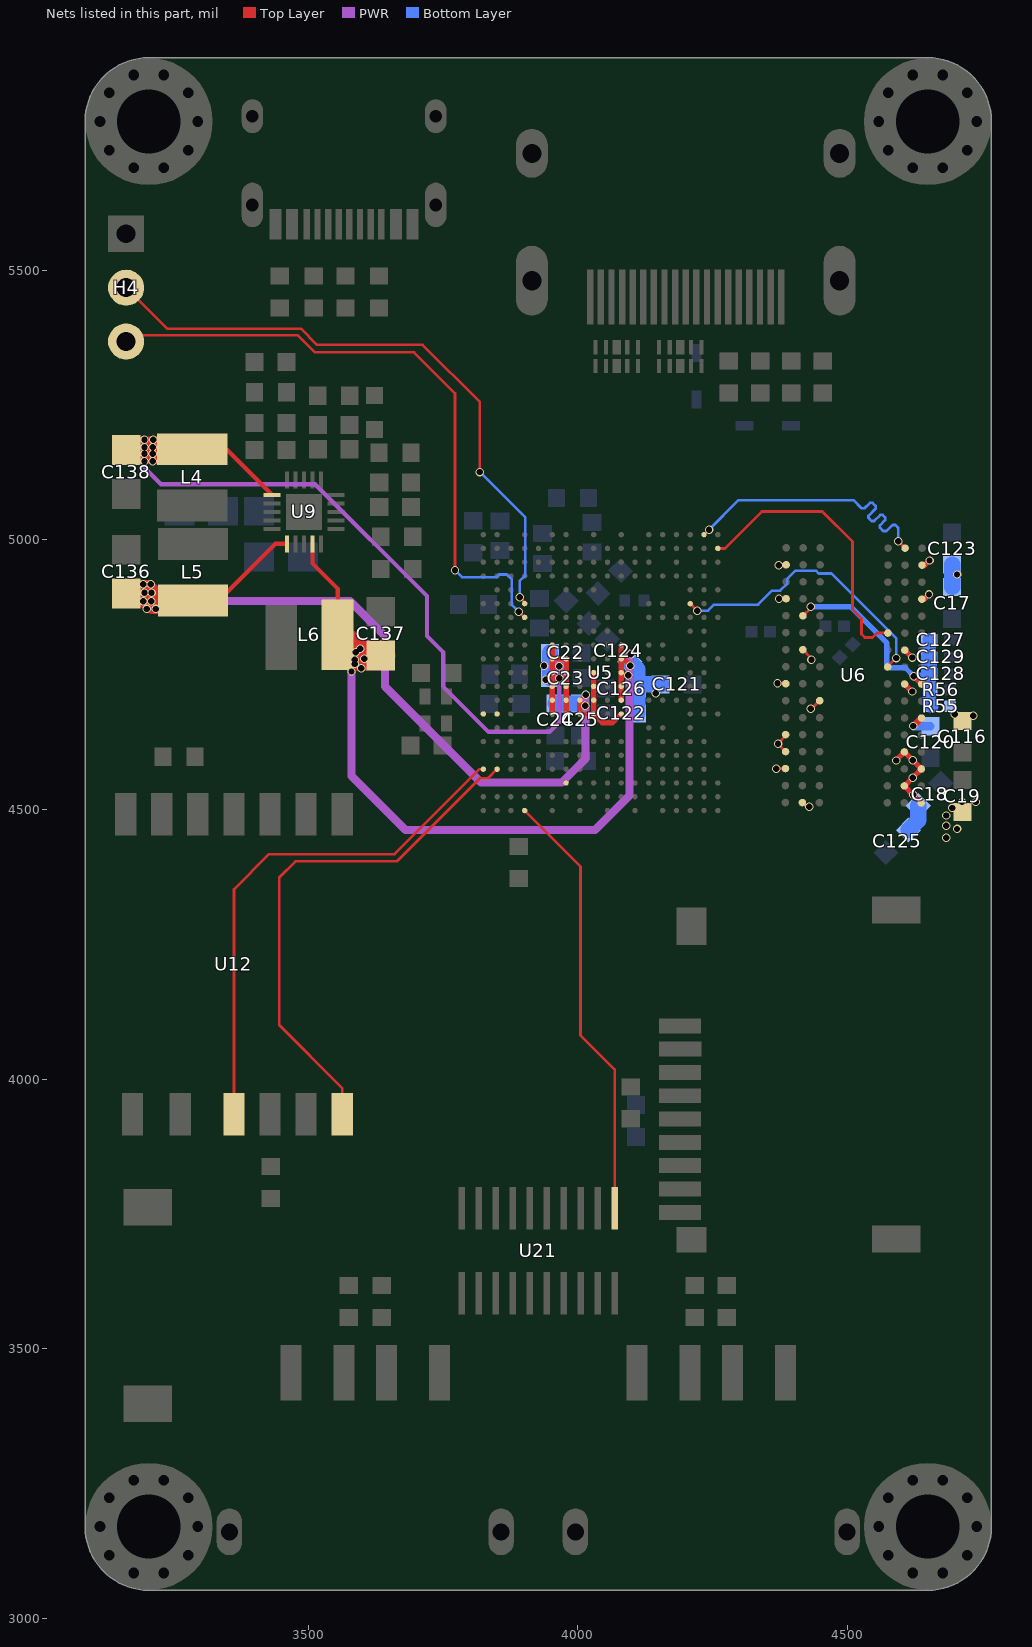
[diagram p0: the nets of this part, all layers, seen from the top]
# Altium PCB MISC105417.pcbdoc (part 5 of 5)
Units mil, origin at the board's own origin, x right, y up, seen from the top; angles counter-clockwise.
Board outline 1681.1 x 2842.52 mil, 4 copper layers (Top Layer, GND, PWR, Bottom Layer), stack 62.447 mil thick; 102 components, 152 nets, 737 pads, 611 vias.

## Via types
v1: diameter 15.7, hole 11.8, Top Layer to Bottom Layer, 611 vias

## Nets (pads, with @x,y where several pads share a name; then routed paths per layer and width w, separated by ;. In a path a pad name is that pad's centre, name@x,y a point inside that pad or via, vN(x,y) a via of type N, cw(c..) or ccw(c..) an arc to the next point about the centre after c; other vN are vias at no path point) (continued)
SRAS: U5.T16 U6.J3 | length 535
  Top Layer w5: U5.T16@4208.34,4881.95 4221.2,4869.09 v1(4221.2,4868.94) ; U6.J3@4574.64,4764.39 4574.64,4765.38 v1(4590.2,4780.94)
  Bottom Layer w5: v1(4221.2,4868.94) 4241.2,4868.94 4252.2,4879.94 4334.2,4879.94 4360.2,4905.94 4374.94,4905.94 4388.43,4919.43 4388.43,4928.16 4403.36,4943.09 4441.46,4943.09 4446.61,4937.94 4470.2,4937.94 4590.2,4817.94 v1(4590.2,4780.94)
SRST: U5.U21 U6.T2 | length 535
  Top Layer w5: U5.U21@4233.93,5009.91 4242.96,5018.94 v1(4243.2,5018.94) ; v1(4594.2,4997.94) 4606.84,4985.31 U6.T2@4606.84,4984.79
  Bottom Layer w5: v1(4243.2,5018.94) 4298.2,5073.94 4511.13,5073.94 4526.29,5058.78 4531.81,5058.78 4541.8,5068.78 4546.37,5068.78 4552.2,5062.94 4552.2,5057.94 4538.64,5044.37 4538.64,5041.19 4544.55,5035.28 4549.55,5035.28 4560.95,5046.69 4564.95,5046.69 4569.88,5041.76 4569.88,5036.82 4559.99,5026.93 4559.99,5022.87 4566.1,5016.75 4572.22,5016.75 4583.4,5027.93 4588.72,5027.93 4594.2,5022.45 v1(4594.2,4997.94)
STATE_LED: U5.G3
SVREF: C127.2 C128.2 C129.2 R55.2 R56.1 U6.H1 U6.M8 | length 464.4
  Top Layer w5: U6.M8@4417.44,4859.39 4432.2,4874.16 v1(4432.2,4875.94)
  Top Layer w10: v1@4623.29,4746.94 U6.H1@4637.54,4732.69
  Bottom Layer w10: v1(4432.2,4875.94) 4506.2,4875.94 4573.2,4808.94 4573.2,4770.94 4581.19,4762.96 4607.19,4762.96 v1(4623.2,4746.94)
  Bottom Layer w15: v1(4623.2,4746.94) 4646.51,4746.94 C128.2@4651.51,4751.94
  Bottom Layer w25: C128.2@4651.51,4751.94 4651.51,4696.36 R55.2@4655.93,4691.94 ; C129.2@4651.51,4782.94 C127.2@4651.51,4814.66
  Bottom Layer w30: C128.2@4651.51,4751.94 C129.2@4651.51,4782.94
SWE: U5.V20 U6.L3 | length 535
  Top Layer w5: U5.V20@4259.52,4984.31 4272.57,4984.31 4341.2,5052.94 4453.2,5052.94 4509.2,4996.94 4509.2,4870.94 4525.85,4854.29 4525.85,4825.29 4532.2,4818.94 4546.2,4818.94 4554.65,4827.39 U6.L3@4574.84,4827.39
TS_IRQ: U5.D1 U21.11 | length 806.7
  Top Layer w5: U5.D1@3901.25,4498.09 4004.86,4394.48 4004.86,4081.14 4068.17,4017.83 U21.11@4068.17,3760.55
UART0_RX: H4.3 U5.D15 | length 1184.8
  Top Layer w5: H4.3@3162,5368 3174,5380 3480,5380 3512,5348 3696,5348 3772,5272 v1(3772,4944) ; v1(3890.2,4866.94) 3890.67,4866.94 U5.D15@3901.25,4856.36
  Bottom Layer w5: v1(3772,4944) 3785,4931 3849,4931 3854,4936 3868,4936 3877.52,4926.48 3877.52,4879.63 v1(3890.2,4866.94)
UART0_TX: H4.2 U5.D16 | length 1161.1
  Top Layer w5: H4.2@3162,5468 3238,5392 3486,5392 3516,5362 3712,5362 3818,5256 v1(3818,5126) ; v1@3892.05,4894 3901.25,4884.8 U5.D16@3901.25,4881.95
  Bottom Layer w5: v1(3818,5126) 3902.55,5041.45 3902.55,4934.05 3892,4923.5 v1(3892,4894)
UART1_RX: U5.B4 U12.13 | length 974.7
  Top Layer w5: U12.13@3562.72,3934.91 3562.72,3983.28 3446,4100 3446,4374 3476,4404 3664,4404 3818,4558 3833.2,4558 U5.B4@3850.07,4574.87
UART1_TX: U5.A4 U12.10 | length 971.9
  Top Layer w5: U12.10@3361.94,3934.91 3361.94,4351.94 3427.09,4417.09 3659.63,4417.09 3817.41,4574.87 U5.A4@3824.48,4574.87
VCC_DRAM: C17.2 C18.2 C19.2 C116.2 C120.2 C121.2 C122.2 C123.2 C124.2 C125.2 C126.2 C137.2 L6.2 R55.1 U5.L9 U5.L10 U5.L11 U5.L12 U5.L13 U6.A1 U6.A8 U6.B2 U6.C1 U6.C9 U6.D2 U6.D9 U6.E9 U6.F1 U6.G7 U6.H2 U6.H9 U6.K2 U6.K8 U6.N1 U6.N9 U6.R1 U6.R9 U9.4 | length 2179.7
  Top Layer w5: v1@4368.26,4575.99 U6.C9@4385.04,4575.99 ; v1(4370.2,4733.94) 4385.09,4733.94 U6.H9@4385.54,4733.49 ; v1@4372.26,4952.99 4385.24,4952.99 U6.R9@4386.24,4953.99 ; v1(4372.95,4891.23) 4373.19,4890.99 U6.N9@4386.04,4890.99 ; U6.D9@4385.14,4607.49 4371.2,4621.43 v1(4371.2,4621.94) 4385.24,4635.99 U6.E9@4385.24,4638.99 ; U6.A8@4416.34,4512.89 4424.29,4504.94 v1(4429.2,4504.94) ; U6.K8@4417.24,4796.39 4433.2,4780.43 v1(4433.2,4777.94) ; v1(4432.2,4686.94) 4433.59,4686.94 U6.G7@4448.44,4701.79
  Top Layer w8: U9.4@3507.7,4992.9 3507.7,4956.3 3554.28,4909.72 L6.2@3554.28,4824
  Top Layer w10: U5.L9@4080.39,4702.82 U5.L10@4080.39,4728.41 U5.L11@4080.39,4754 ; U5.L13@4080.39,4805.18 U5.L12@4080.39,4779.59 ; v1(4093.2,4748.94) 4085.45,4748.94 U5.L11@4080.39,4754 ; v1(4097.2,4766.94) 4084.56,4779.59 U5.L12@4080.39,4779.59 ; v1(4590.2,4590.94) 4590.2,4591.36 U6.D2@4605.64,4606.79 v1(4620.85,4591.58) 4637.04,4575.39 U6.C1@4637.04,4575.19 v1(4621.05,4559.21) 4605.64,4543.79 U6.B2@4605.44,4543.79 4605.44,4543.59 v1(4621.68,4527.35) U6.A1@4636.84,4512.19 ; U6.H2@4606.04,4732.79 4619.89,4718.94 v1(4620.2,4718.94) ; U6.K2@4606.24,4795.79 4620.09,4781.94 v1(4620.2,4781.94) ; U6.N1@4638.04,4890.19 4642.45,4890.19 v1(4651.2,4898.94) ; U6.R1@4638.24,4953.19 4643.45,4953.19 v1(4652.2,4961.94) ; U5.L11@4080.39,4754 U5.L12@4080.39,4779.59
  Top Layer w12: v1(4622.2,4654.94) 4622.59,4654.94 U6.F1@4637.34,4669.69
  Top Layer w55: L6.2@3554.28,4824 3592.54,4785.74 C137.2@3634.16,4785.74
  PWR w15: v1(3586,4770) 3580,4764 v1(3580,4756) 3580,4562 3680,4462 4032,4462 4096,4526 4096,4785.74 v1(4098.2,4787.94)
  Bottom Layer w10: v1(4097.2,4766.94) C124.2@4097.2,4772.94
  Bottom Layer w15: v1(4622.2,4654.94) 4622.68,4654.47 C120.2@4654.2,4654.47
  Bottom Layer w30: C124.2@4096.08,4774.06 4097.2,4772.94 4110,4760.15 C126.2@4110,4724.21 ; C122.2@4110,4678.21 C126.2@4110,4724.21 ; C121.2@4153.54,4732.31 4118.1,4732.31 C126.2@4110,4724.21 ; C125.2@4613.17,4461.88 4631.33,4480.04 C18.2@4631.33,4507.06 ; C17.2@4694.2,4912.47 C123.2@4694.2,4954.41
  other v1: 4683.2,4447.45 4703.2,4463.94 4683.2,4469.79 4683.2,4488.94 4694.2,4502.94 4712.47,4513.94 4738.2,4513.94 4368.2,4575.94 4733.2,4673.94 4699.2,4676.94 4144.2,4715.94 3598,4762 3586,4778 3604,4780 3588,4792 3596,4798 4703.2,4935.94 4372.2,4952.94
VDD_CPU: C24.2 C25.2 C136.1 L5.2 U5.H8 U5.H9 U5.J8 U5.J9 U5.J10 U5.J11 U5.L8 U9.1 | length 1792.2
  Top Layer w5: v1(4013.73,4692.23) 4013.73,4692.7 U5.H9@4003.61,4702.82 4013.73,4712.94 v1(4014.2,4712.94)
  Top Layer w8: L5.2@3286,4887.72 3333.72,4887.72 3438.9,4992.9 U9.1@3460.5,4992.9
  Top Layer w10: U5.H9@4003.61,4702.82 U5.H8@4003.61,4677.23 U5.J8@4029.2,4677.23 ; U5.J11@4029.2,4754 U5.J10@4029.2,4728.41 U5.J9@4029.2,4702.82 U5.J8@4029.2,4677.23 ; U5.L8@4080.39,4677.23 4064.1,4660.94 4045.49,4660.94 U5.J8@4029.2,4677.23
  Top Layer w50: C136.1@3162.16,4900.74 3199.26,4900.74 3212.28,4887.72 L5.2@3286,4887.72
  PWR w15: v1(3196,4902) v1(3209.17,4902) 3224.17,4887 3577,4887 3642,4822 3642,4728 3820,4550 3970,4550 4014.2,4594.2 v1(4014.2,4712.94)
  Bottom Layer w5: C25.2@4004.25,4696.51 4014.2,4706.47 v1(4014.2,4712.94)
  Bottom Layer w30: C24.2@3958.2,4696.51 C25.2@4004.25,4696.51
  other v1: 3200,4872 3216.68,4872 3194,4886 3208.56,4886 3194,4918 3207.95,4918
VDD_GPU: C22.2 C23.2 C138.1 L4.2 U5.F8 U5.F9 U5.F10 U5.F11 U5.F12 U5.F13 U5.G8 U5.G9 U5.G10 U5.G11 U5.G12 U9.16 | length 1825.5
  Top Layer w8: L4.2@3285,5168.28 3348.12,5168.28 U9.16@3432.9,5083.5
  Top Layer w10: U5.F8@3952.43,4677.23 U5.F9@3952.43,4702.82 U5.F10@3952.43,4728.41 U5.F11@3952.43,4754 U5.F12@3952.43,4779.59 ; U5.F13@3952.43,4805.18 U5.F12@3952.43,4779.59 ; U5.G8@3978.02,4677.23 U5.G9@3978.02,4702.82 U5.G10@3978.02,4728.41 U5.G11@3978.02,4754 U5.G12@3978.02,4779.59 U5.F12@3952.43,4779.59
  Top Layer w50: C138.1@3162.16,5166.55 3283.27,5166.55 L4.2@3285,5168.28
  PWR w8: v1(3196,5186) v1(3196,5172) v1(3196,5160) v1(3196,5146) 3196,5134 3226.5,5103.5 3512.5,5103.5 3720,4896 3720,4822 3750,4792 3750,4728 3834,4644 3947.01,4644 3965.2,4662.2 v1(3965.2,4743.21)
  PWR w25: v1(3965.2,4743.21) v1(3965.2,4765.94)
  Bottom Layer w30: C23.2@3947.96,4743.94 C22.2@3947.96,4790.68
  other v1: 3940.2,4740.94 3937.2,4766.94 3211.68,5146 3211.55,5160 3211.14,5172 3212.09,5186
WIFI_AP: U5.B8
WIFI_AP2: U5.A8
pads on no net: U5.A2 U5.A19 U5.A20 U5.B1 U5.B2 U5.B3 U5.B9 U5.B10 U5.B20 U5.B21 U5.C2 U5.C3 U5.C4 U5.C8 U5.C9 U5.C10 U5.C11 U5.C16 U5.D3 U5.D4 U5.D5 U5.D14 U5.E2 U5.E3 U5.E4 U5.E5 U5.E6 U5.F1 U5.F2 U5.F3 U5.F4 U5.G2 U5.G4 U5.G5 U5.G6 U5.G19 U5.G20 U5.H1 U5.H2 U5.H3 U5.H4 U5.H5 U5.H6 U5.J21 U5.K4 U5.K5 U5.K6 U5.L4 U5.L5 U5.L6 U5.L18 U5.L19 U5.L20 U5.N7 U5.N10 U5.P7 U5.P9 U5.P10 U5.P12 U5.R9 U5.R12 U5.T5 U5.T6 U5.T7 U5.T9 U5.T11 U5.T12 U5.U5 U5.U8 U5.U9 U5.U10 U5.U11 U5.U12 U5.V8 U5.V10 U9.10 U9.14 U22.2 USB3.A8 USB3.B8 USB10.14

## Polygon pours and split planes (outlines as drawn)
VDD_GPU on Top Layer (solid, remove dead copper, pour order 6): 3988.2,4783.94 3988.2,4673.94 3983.2,4668.94 3938.2,4668.94 3933.2,4673.94 3933.2,4808.94 3938.2,4813.94 3963.2,4813.94 3988.2,4788.94
1V8 on Top Layer (solid, remove dead copper, pour order 8): 3923.2,4738.94 3918.2,4733.94 3908.2,4733.94 3893.2,4748.94 3893.2,4783.94 3898.2,4788.94 3918.2,4788.94 3923.2,4783.94
3V3 on Top Layer (solid, remove dead copper, pour order 10): 3908.2,4733.94 3908.2,4698.94 3938.2,4668.94 4008.2,4668.94 4048.2,4628.94 4048.2,4593.94 4043.2,4588.94 4018.2,4588.94 4013.2,4593.94 4013.2,4623.94 3998.2,4638.94 3973.2,4638.94 3963.2,4628.94 3963.2,4593.94 3958.2,4588.94 3943.2,4588.94 3938.2,4593.94 3938.2,4633.94 3933.2,4638.94 3898.2,4638.94 3883.2,4653.94 3883.2,4728.94 3888.2,4733.94
1V8 on Bottom Layer (solid, remove dead copper, pour order 58): 3923.2,4768.94 3923.2,4738.94 3913.2,4728.94 3878.2,4728.94 3873.2,4733.94 3873.2,4768.94 3878.2,4773.94 3918.2,4773.94
3V3 on Bottom Layer (solid, remove dead copper, pour order 60): 3913.2,4718.94 3913.2,4673.94 3893.2,4653.94 3878.2,4653.94 3873.2,4658.94 3873.2,4718.94 3878.2,4723.94 3908.2,4723.94
GND on Top Layer (solid, remove dead copper, pour order 16): 4063.2,4673.94 4058.2,4668.94 4048.2,4668.94 4038.2,4678.94 4038.2,4758.94 4033.2,4763.94 4018.2,4763.94 4013.2,4758.94 4013.2,4723.94 4008.2,4718.94 3998.2,4718.94 3993.2,4723.94 3993.2,4783.94 3958.2,4818.94 3948.2,4818.94 3943.2,4823.94 3943.2,4863.94 3948.2,4868.94 4058.2,4868.94 4063.2,4863.94
VDD_CPU on Top Layer (solid, remove dead copper, pour order 18): 4088.2,4683.94 4088.2,4663.94 4073.2,4648.94 4028.2,4648.94 4008.2,4668.94 3993.2,4668.94 3993.2,4718.94 4008.2,4718.94 4013.2,4723.94 4018.2,4723.94 4018.2,4763.94 4033.2,4763.94 4038.2,4758.94 4038.2,4678.94 4048.2,4668.94 4058.2,4668.94 4068.2,4678.94 4068.2,4683.94 4073.2,4688.94 4083.2,4688.94
1V8 on Top Layer (solid, remove dead copper, pour order 20): 4064.2,4874.94 4058.2,4868.94 3960.2,4868.94 3954.2,4874.94 3954.2,4886.94 3960.2,4892.94 3976.2,4892.94 3998.2,4914.94 4010.2,4914.94 4024.2,4900.94 4060.2,4900.94 4064.2,4896.94
VCC_DRAM on PWR (solid, remove dead copper): 3602,4810 3614,4798 3614,4562 3690,4486 4005.05,4486 4073.05,4554 4111.82,4554 4260.91,4404.91 4194,4338 3610,4338 3518,4430 3518,4795.78 3534.76,4810
VDD_CPU on PWR (solid, remove dead copper): 3602,4958 3686,4874 3686,4742 3836,4592 3950,4592 3986,4628 3986,4710 3996,4720 4048,4720 4065.2,4702.8 4065.2,4545.2 4006,4486 3689.28,4486 3614,4561.28 3614,4798 3602,4810 3204,4810 3158,4856 3158,4920 3196,4958
VDD_GPU on PWR (solid, remove dead copper): 3346,5200 3370,5176 3532,5176 3802,4906 3802,4704 3844,4662 3908,4662 3926,4680 3926,4769.72 3937.2,4780.92 3986,4780.92 3986,4628 3950,4592 3836,4592 3686,4742 3686,4874 3602,4958 3196,4958 3178,4976 3178,5190 3188,5200
1V8 on PWR (solid, remove dead copper): 3916,5102 4006,5012 4006,4994 3998,4986 3976,4986 3956,4966 3956,4920.5 3978.5,4898 4004,4898 4010,4892 4010,4840 3950.92,4780.92 3937.2,4780.92 3926,4769.72 3926,4728 3920,4722 3894,4722 3890,4726 3890,4826 3922,4858 3922,4998 3902,5018 3756,5018 3710,5064 3710,5093.75 3718.25,5102
VCC_DRAM on PWR (solid, remove dead copper): 4748.2,5008.94 4748.2,4488.94 4658.2,4398.94 4148.2,4398.94 4064.48,4482.67 4064.48,5015.22 4208.2,5158.94 4598.2,5158.94
$2N1522 on Top Layer (solid, remove dead copper, pour order 32): 3416,4886 3416,4892 3484,4960 3484,5010 3486,5012 3498,5012 3500,5010 3500,4908 3482,4890 3482,4760 3478,4756 3420,4756 3416,4760
VCC_DRAM on Top Layer (solid, remove dead copper, pour order 34): 3500,5010 3502,5012 3514.38,5012 3516,5010.38 3516,4974 3586,4904 3586,4838 3584,4836 3524,4836 3522,4838 3522,4890 3500,4912
VDD_CPU on Top Layer (solid, remove dead copper, pour order 36): 3216,4918 3340,4918
VDD_CPU on Top Layer (solid, remove dead copper, pour order 38): 3340,4918 3344.5,4918 3434.5,5008 3464,5008 3464,4982 3444,4962 3436,4962 3430,4956 3430,4908 3380,4858 3350,4858 3342,4866 3340,4866
PS on Top Layer (solid, remove dead copper, pour order 40): 3468,5010 3482,5010 3484,5008 3484,4960 3452,4928 3438,4928 3430,4936 3430,4956 3436,4962 3450,4962 3466,4978 3466,5008
PS on Top Layer (solid, remove dead copper, pour order 42): 3450,5026 3452,5024 3452,5012 3450,5010 3434,5010 3422,4998 3400,4998 3396,5002 3396,5019.74 3402.26,5026
$2N1523 on Top Layer (solid, remove dead copper, pour order 44): 3338,5022 3356,5022 3376,5042 3450,5042 3452,5040 3452,5032 3450,5030 3406,5030 3392,5016 3392,4986 3370,4964 3333.98,4964 3327.98,4970 3326,4970 3326,5010
VDD_GPU on Top Layer (solid, remove dead copper, pour order 46): 3330,5200 3366,5200 3380,5186 3380,5152 3388,5144 3412,5144 3448,5108 3448,5080 3446,5078 3422,5078 3420,5080 3404,5080 3345.4,5138.6 3337.4,5138.6 3330,5146
$2N1524 on Top Layer (solid, remove dead copper, pour order 48): 3338.03,5092 3362,5092 3394,5060 3450,5060 3452,5058 3452,5048 3450,5046 3376,5046 3364,5034 3334.72,5034 3334.72,5088.69
PS on Top Layer (solid, remove dead copper, pour order 50): 3396,5088 3408,5076 3448,5076 3450,5074 3450,5062 3448,5060 3394,5060 3378,5076 3390,5088
1V8 on Top Layer (solid, remove dead copper, pour order 52): 3443.54,5166.27 3477.02,5166.27 3477.02,5137.02 3468,5128 3468,5096 3466,5094 3454,5094 3452,5096 3452,5110 3438,5124 3438,5164 3442,5168 3443.54,5166.46
3V3 on Top Layer (solid, remove dead copper, pour order 54): 3497.18,5169.02 3534.98,5169.02 3538,5166 3538,5146 3516.32,5124.32 3516.32,5092.32 3514,5090 3502,5090 3500,5092 3500,5140 3494,5146 3494,5166 3496,5168
PS on Bottom Layer (solid, remove dead copper, pour order 102): 3640,5672 3650,5662 3650,5612 3642,5604 3564,5604 3394,5434 3394,5162 3449.19,5106.81 3449.19,4907.19 3442,4900 3442,3976 3556,3862 3556,3784 3538,3766 3512,3766 3312,3966 3312,5472.78 3511.22,5672
PS on Top Layer (solid, remove dead copper, pour order 58): 3542,3830 3550,3822 3550,3698 3496,3644 3496,3490 3438,3490 3438,3698 3492,3752 3492,3820 3502,3830
PS on Bottom Layer (solid, remove dead copper, pour order 106): 3608,5672 3684.41,5672 3701.26,5655.15 3701.26,5574.74 3714,5562 3746,5562 3822,5638 4016,5638 4164,5490 4164,5274 4198,5240 4326,5240 4332,5234 4332,5202 4318,5188 4144,5188 4072,5260 4072,5452 3990,5534 3876,5534 3824,5482 3662,5482 3614,5530 3614,5586 3576.76,5623.24 3576.76,5640.76
3V3 on PWR (solid, remove dead copper): 3000,5970 3000,3000 4850,3000 4850,5970
GND on Top Layer (solid, remove dead copper, pour order 64): 3000,5970 3000,3000 4850,3000 4850,5970
GND on Bottom Layer (solid, remove dead copper, pour order 112): 3000,5970 3000,3000 4850,3000 4850,5970
3V3 on Top Layer (solid, remove dead copper, pour order 0): 3875.28,3654 3946,3654 3952,3648 3952,3563 3949,3560 3873,3560 3869,3564 3869,3647.72
PS on Top Layer (solid, remove dead copper, pour order 2): 3969,3654 4071,3654 4139,3586 4139,3336 4084.67,3281.67 3503.33,3281.67 3437,3348 3437,3508 3444,3515 3489,3515 3496,3508 3496,3387 3527,3356 3919,3356 3954,3391 3954,3639
GND on Top Layer (solid, remove dead copper, pour order 4): 3780.79,3654 3851.51,3654 3857.51,3648 3857.51,3563 3854.51,3560 3778.51,3560 3774.51,3564 3774.51,3647.72

## Keep-outs
Top Layer:
  region: 4543.2,5158.94 4693.2,5008.94 4693.2,4523.94 4568.2,4398.94 4148.2,4398.94 4063.2,4483.94 4063.2,4638.94 4088.2,4663.94 4088.2,4683.94 4083.2,4688.94 4063.2,4688.94 4063.2,5013.94 4208.2,5158.94
  region: 3482,4890 3482,4756 3524,4756 3524,4890
  region: 3216,4962 3216,4918 3350,4918 3350,4962
  region: 3215.68,5138.6 3215.68,5092 3352,5092 3352,5138.6
  region: 3076,3894 3192,3894 3196,3898 3196,3996 3208,4008 3312,4008 3324,3996 3324,3182 3076,3182
PWR:
  region: 3076,3894 3192,3894 3196,3898 3196,3996 3208,4008 3312,4008 3324,3996 3324,3182 3076,3182
Bottom Layer:
  region: 4653.2,4523.94 4543.2,4413.94 4178.2,4413.94 4073.2,4518.94 4073.2,4978.94 4228.2,5133.94 4567.59,5133.94 4653.2,5048.33
  region: 3076,3894 3192,3894 3196,3898 3196,3996 3208,4008 3312,4008 3324,3996 3324,3182 3076,3182
GND:
  region: 3076,3894 3192,3894 3196,3898 3196,3996 3208,4008 3312,4008 3324,3996 3324,3182 3076,3182
Board Outline Layer:
  the board outline again, w10

## Silkscreen, mask and mechanical layers (free items; w line width, h text height)
Top Silkscreen Layer:
  text "GND" at 3222.97,5534.68 h60
  text "TXD" at 3220.97,5434.68 h60
  text "RXD" at 3226.97,5334.68 h60
  text "Cannot be reinstalled, right!" at 4480.2,4966.94 h70 r270
  text "H616_Board_V1.3" at 3617,4137 h60
  text "2024-4-15" at 3704,4057 h60